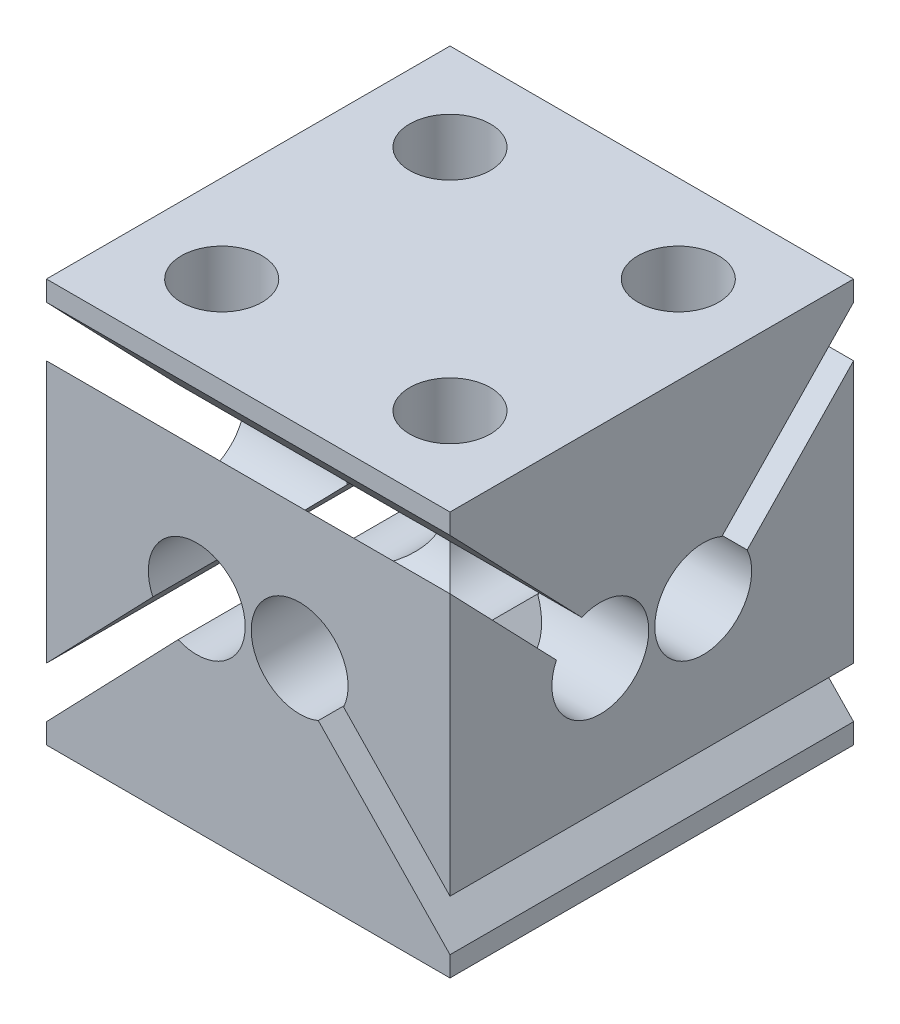
from build123d import *

# Parameters (mm, degrees)
SKETCH1_W           = 10
SKETCH1_H           = 10
BOSS_EXTRUDE1_DEPTH = 10
CUT_EXTRUDE1_DEPTH  = 16
CUT_EXTRUDE2_DEPTH  = 16
SKETCH5_R           = 0.6
CUT_EXTRUDE3_DEPTH  = 2
SKETCH6_R           = 1
CUT_EXTRUDE4_DEPTH  = 1.5


with BuildPart() as part:
    # Sketch1 → Boss-Extrude1 (new body)
    with BuildSketch(Plane(origin=(0, 0, 0), x_dir=(1, 0, 0), z_dir=(0, 1, 0))):
        Rectangle(SKETCH1_W, SKETCH1_H)
    extrude(amount=BOSS_EXTRUDE1_DEPTH)

    # Sketch2 → Cut-Extrude1 (cut, through all)
    with BuildSketch(Plane.XY.offset(5)):
        with BuildLine():
            Line((2.363818154, 4.495544821), (5, 1.754964793))
            Line((5, 1.754964793), (5, 0.5))
            Line((5, 0.5), (1.736808704, 3.892420332))
            ThreePointArc((1.736808704, 3.892420332), (0.443104153, 5.864840621), (2.363818154, 4.495544821))
        make_face()
        with BuildLine():
            Line((-5, 1.754964793), (-5, 0.5))
            Line((-5, 0.5), (-1.736808704, 3.892420332))
            ThreePointArc((-1.736808704, 3.892420332), (-0.443104153, 5.864840621), (-2.363818154, 4.495544821))
            Line((-2.363818154, 4.495544821), (-5, 1.754964793))
        make_face()
    extrude(amount=-CUT_EXTRUDE1_DEPTH, mode=Mode.SUBTRACT)

    # Sketch3 → Cut-Extrude2 (cut, through all)
    with BuildSketch(Plane(origin=(5, 0, 0), x_dir=(0, 0, -1), z_dir=(1, 0, 0))):
        with BuildLine():
            Line((2.363818154, 5.504455179), (5, 8.245035207))
            Line((5, 8.245035207), (5, 9.5))
            Line((5, 9.5), (1.736808704, 6.107579668))
            ThreePointArc((1.736808704, 6.107579668), (0.443104153, 4.135159379), (2.363818154, 5.504455179))
        make_face()
        with BuildLine():
            Line((-5, 9.5), (-5, 8.245035207))
            Line((-5, 8.245035207), (-2.363818154, 5.504455179))
            ThreePointArc((-2.363818154, 5.504455179), (-0.443104153, 4.135159379), (-1.736808704, 6.107579668))
            Line((-1.736808704, 6.107579668), (-5, 9.5))
        make_face()
    extrude(amount=-CUT_EXTRUDE2_DEPTH, mode=Mode.SUBTRACT)

    # Sketch5 → Cut-Extrude3 (cut)
    with BuildSketch(Plane.XZ):
        with Locations(Location((-2.84590029, 2.810845343, 0), (0, 0, 270))):
            Circle(SKETCH5_R)
        with Locations(Location((2.84590029, -2.810845343, 0), (0, 0, 270))):
            Circle(SKETCH5_R)
    extrude(amount=-CUT_EXTRUDE3_DEPTH, mode=Mode.SUBTRACT)

    # Sketch6 → Cut-Extrude4 (cut)
    with BuildSketch(Plane(origin=(0, 10, 0), x_dir=(1, 0, 0), z_dir=(0, 1, 0))):
        with Locations(Location((-2.828427125, 2.828427125, 0), (0, 0, 270))):
            Circle(SKETCH6_R)
        with Locations(Location((2.828427125, 2.828427125, 0), (0, 0, 270))):
            Circle(SKETCH6_R)
        with Locations(Location((2.828427125, -2.828427125, 0), (0, 0, 270))):
            Circle(SKETCH6_R)
        with Locations(Location((-2.828427125, -2.828427125, 0), (0, 0, 270))):
            Circle(SKETCH6_R)
    extrude(amount=-CUT_EXTRUDE4_DEPTH, mode=Mode.SUBTRACT)


solid = part.part
